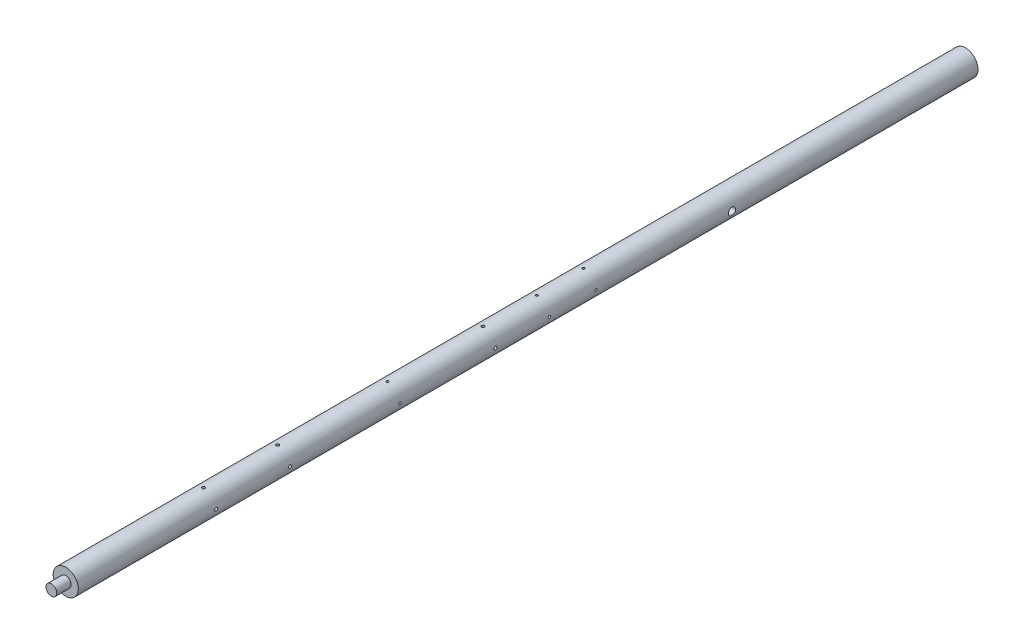
from build123d import *

# Parameters (mm, degrees)
SKETCH_1_R               = 17.5
EXTRUDE_1_DEPTH          = 1313
SKETCH_2_R               = 7.5
EXTRUDE_2_DEPTH          = 10
CHAMFER_1_SIZE           = 1
SKETCH_3_R               = 5
CUT_EXTRUDE_1_DEPTH      = 20
PATTERN_CIRCULAR_1_COUNT = 4
PATTERN_LINEAR_1_COUNT   = 2
PATTERN_LINEAR_1_PITCH   = 65
PATTERN_CIRCULAR_2_COUNT = 4
PATTERN_LINEAR_2_COUNT   = 2
PATTERN_LINEAR_2_PITCH   = 273
PATTERN_LINEAR_3_COUNT   = 2
PATTERN_LINEAR_3_PITCH   = 286
PATTERN_LINEAR_4_COUNT   = 2
PATTERN_LINEAR_4_PITCH   = 389
CUT_EXTRUDE_START        = -90
SKETCH_9_R               = 17.5
SKETCH_9_R_2             = 7.5
CUT_EXTRUDE_2_DEPTH      = 90
SKETCH_10_R              = 8.093395995
CUT_EXTRUDE_3_DEPTH      = 80
EXTRUDE_START            = 30
SKETCH_11_R              = 17.5
EXTRUDE_3_DEPTH          = 30


with BuildPart() as part:
    # 草图1 → 凸台-拉伸1 (new body)
    with BuildSketch(Plane.XY):
        Circle(SKETCH_1_R)
    extrude(amount=EXTRUDE_1_DEPTH)

    # 草图2 → 凸台-拉伸2 (add)
    with BuildSketch(Plane.XY.offset(1313)):
        Circle(SKETCH_2_R)
    extrude(amount=EXTRUDE_2_DEPTH)

    # 倒角1
    chamfer_1_edges = [part.edges().sort_by_distance(p)[0] for p in [
        (-7.5, 0, 1323),
    ]]
    chamfer(chamfer_1_edges, length=CHAMFER_1_SIZE)

    # 草图3 → 切除-拉伸1 (cut, symmetric)
    with BuildSketch(Plane(origin=(0, 0, 0), x_dir=(0, 0, -1), z_dir=(1, 0, 0))):
        with Locations(Location((-312.5, 0, 0), (0, 0, 180))):
            Circle(SKETCH_3_R)
    extrude(amount=CUT_EXTRUDE_1_DEPTH, both=True, mode=Mode.SUBTRACT)

    # 草图5 → M4x0.7 螺纹孔1 (revolve, cut)
    with BuildSketch(Plane(origin=(17.5, 0, 502), x_dir=(0, 0, -1), z_dir=(0, 1, 0))):
        Polygon((0, 0), (0, 11.091420021), (1.65, 10.1), (1.65, 0), align=None)
    m4x0_7_1 = revolve(axis=Axis((23.85, 0, 502), (-1, 0, 0)), mode=Mode.SUBTRACT)

    # 阵列(圆周)1: M4x0.7 螺纹孔1 ×4 about axis
    pattern_circular_1_axis = Axis((0, 0, 1313), (0, 0, -1))
    for i in range(1, PATTERN_CIRCULAR_1_COUNT):
        add(m4x0_7_1.rotate(pattern_circular_1_axis, i * 360 / PATTERN_CIRCULAR_1_COUNT), mode=Mode.SUBTRACT)

    # 阵列(线性)1: M4x0.7 螺纹孔1 ×2
    with Locations(*[(0, 0, i * PATTERN_LINEAR_1_PITCH) for i in range(1, PATTERN_LINEAR_1_COUNT)]):
        add(m4x0_7_1, mode=Mode.SUBTRACT)

    # 阵列(线性)1 copy 1 sketch → 阵列(线性)1 copy 1 (revolve, cut)
    with BuildSketch(Plane(origin=(0, -17.5, 567), x_dir=(0, 0, -1), z_dir=(1, 0, 0))):
        Polygon((0, 0), (0, 11.091420021), (1.65, 10.1), (1.65, 0), align=None)
    revolve(axis=Axis((0, -23.85, 567), (0, 1, 0)), mode=Mode.SUBTRACT)

    # 阵列(线性)1 copy 2 sketch → 阵列(线性)1 copy 2 (revolve, cut)
    with BuildSketch(Plane(origin=(-17.5, 0, 567), x_dir=(0, 0, -1), z_dir=(0, -1, 0))):
        Polygon((0, 0), (0, 11.091420021), (1.65, 10.1), (1.65, 0), align=None)
    revolve(axis=Axis((-23.85, 0, 567), (1, 0, 0)), mode=Mode.SUBTRACT)

    # 阵列(线性)1 copy 3 sketch → 阵列(线性)1 copy 3 (revolve, cut)
    with BuildSketch(Plane(origin=(0, 17.5, 567), x_dir=(0, 0, -1), z_dir=(-1, 0, 0))):
        Polygon((0, 0), (0, 11.091420021), (1.65, 10.1), (1.65, 0), align=None)
    revolve(axis=Axis((0, 23.85, 567), (0, -1, 0)), mode=Mode.SUBTRACT)

    # 草图8 → M5x0.8 螺纹孔1 (revolve, cut)
    with BuildSketch(Plane(origin=(17.5, 0, 642), x_dir=(0, 0, -1), z_dir=(0, 1, 0))):
        Polygon((0, 0), (0, 13.6618073), (2.1, 12.4), (2.1, 0), align=None)
    m5x0_8_1 = revolve(axis=Axis((23.85, 0, 642), (-1, 0, 0)), mode=Mode.SUBTRACT)

    # 阵列(圆周)2: M5x0.8 螺纹孔1 ×4 about axis
    pattern_circular_2_axis = Axis((0, 0, 1313), (0, 0, -1))
    for i in range(1, PATTERN_CIRCULAR_2_COUNT):
        add(m5x0_8_1.rotate(pattern_circular_2_axis, i * 360 / PATTERN_CIRCULAR_2_COUNT), mode=Mode.SUBTRACT)

    # 阵列(线性)2: M4x0.7 螺纹孔1 ×2
    with Locations(*[(0, 0, i * PATTERN_LINEAR_2_PITCH) for i in range(1, PATTERN_LINEAR_2_COUNT)]):
        add(m4x0_7_1, mode=Mode.SUBTRACT)

    # 阵列(线性)2 copy 1 sketch → 阵列(线性)2 copy 1 (revolve, cut)
    with BuildSketch(Plane(origin=(0, -17.5, 775), x_dir=(0, 0, -1), z_dir=(1, 0, 0))):
        Polygon((0, 0), (0, 11.091420021), (1.65, 10.1), (1.65, 0), align=None)
    revolve(axis=Axis((0, -23.85, 775), (0, 1, 0)), mode=Mode.SUBTRACT)

    # 阵列(线性)2 copy 2 sketch → 阵列(线性)2 copy 2 (revolve, cut)
    with BuildSketch(Plane(origin=(-17.5, 0, 775), x_dir=(0, 0, -1), z_dir=(0, -1, 0))):
        Polygon((0, 0), (0, 11.091420021), (1.65, 10.1), (1.65, 0), align=None)
    revolve(axis=Axis((-23.85, 0, 775), (1, 0, 0)), mode=Mode.SUBTRACT)

    # 阵列(线性)2 copy 3 sketch → 阵列(线性)2 copy 3 (revolve, cut)
    with BuildSketch(Plane(origin=(0, 17.5, 775), x_dir=(0, 0, -1), z_dir=(-1, 0, 0))):
        Polygon((0, 0), (0, 11.091420021), (1.65, 10.1), (1.65, 0), align=None)
    revolve(axis=Axis((0, 23.85, 775), (0, -1, 0)), mode=Mode.SUBTRACT)

    # 阵列(线性)3: M5x0.8 螺纹孔1 ×2
    with Locations(*[(0, 0, i * PATTERN_LINEAR_3_PITCH) for i in range(1, PATTERN_LINEAR_3_COUNT)]):
        add(m5x0_8_1, mode=Mode.SUBTRACT)

    # 阵列(线性)3 copy 1 sketch → 阵列(线性)3 copy 1 (revolve, cut)
    with BuildSketch(Plane(origin=(0, -17.5, 928), x_dir=(0, 0, -1), z_dir=(1, 0, 0))):
        Polygon((0, 0), (0, 13.6618073), (2.1, 12.4), (2.1, 0), align=None)
    revolve(axis=Axis((0, -23.85, 928), (0, 1, 0)), mode=Mode.SUBTRACT)

    # 阵列(线性)3 copy 2 sketch → 阵列(线性)3 copy 2 (revolve, cut)
    with BuildSketch(Plane(origin=(-17.5, 0, 928), x_dir=(0, 0, -1), z_dir=(0, -1, 0))):
        Polygon((0, 0), (0, 13.6618073), (2.1, 12.4), (2.1, 0), align=None)
    revolve(axis=Axis((-23.85, 0, 928), (1, 0, 0)), mode=Mode.SUBTRACT)

    # 阵列(线性)3 copy 3 sketch → 阵列(线性)3 copy 3 (revolve, cut)
    with BuildSketch(Plane(origin=(0, 17.5, 928), x_dir=(0, 0, -1), z_dir=(-1, 0, 0))):
        Polygon((0, 0), (0, 13.6618073), (2.1, 12.4), (2.1, 0), align=None)
    revolve(axis=Axis((0, 23.85, 928), (0, -1, 0)), mode=Mode.SUBTRACT)

    # 阵列(线性)4: M5x0.8 螺纹孔1 ×2
    with Locations(*[(0, 0, i * PATTERN_LINEAR_4_PITCH) for i in range(1, PATTERN_LINEAR_4_COUNT)]):
        add(m5x0_8_1, mode=Mode.SUBTRACT)

    # 阵列(线性)4 copy 1 sketch → 阵列(线性)4 copy 1 (revolve, cut)
    with BuildSketch(Plane(origin=(0, -17.5, 1031), x_dir=(0, 0, -1), z_dir=(1, 0, 0))):
        Polygon((0, 0), (0, 13.6618073), (2.1, 12.4), (2.1, 0), align=None)
    revolve(axis=Axis((0, -23.85, 1031), (0, 1, 0)), mode=Mode.SUBTRACT)

    # 阵列(线性)4 copy 2 sketch → 阵列(线性)4 copy 2 (revolve, cut)
    with BuildSketch(Plane(origin=(-17.5, 0, 1031), x_dir=(0, 0, -1), z_dir=(0, -1, 0))):
        Polygon((0, 0), (0, 13.6618073), (2.1, 12.4), (2.1, 0), align=None)
    revolve(axis=Axis((-23.85, 0, 1031), (1, 0, 0)), mode=Mode.SUBTRACT)

    # 阵列(线性)4 copy 3 sketch → 阵列(线性)4 copy 3 (revolve, cut)
    with BuildSketch(Plane(origin=(0, 17.5, 1031), x_dir=(0, 0, -1), z_dir=(-1, 0, 0))):
        Polygon((0, 0), (0, 13.6618073), (2.1, 12.4), (2.1, 0), align=None)
    revolve(axis=Axis((0, 23.85, 1031), (0, -1, 0)), mode=Mode.SUBTRACT)

    # 草图9 → 切除-拉伸2 (cut)
    with BuildSketch(Plane.XY.offset(1313).offset(CUT_EXTRUDE_START)):
        Circle(SKETCH_9_R)
        Circle(SKETCH_9_R_2, mode=Mode.SUBTRACT)
    extrude(amount=CUT_EXTRUDE_2_DEPTH, mode=Mode.SUBTRACT)

    # 草图10 → 切除-拉伸3 (cut)
    with BuildSketch(Plane.XY.offset(1323)):
        Circle(SKETCH_10_R)
    extrude(amount=-CUT_EXTRUDE_3_DEPTH, mode=Mode.SUBTRACT)

    # 草图11 → 凸台-拉伸3 (add)
    with BuildSketch(Plane(origin=(0, 0, 0), x_dir=(-1, 0, 0), z_dir=(0, 0, -1)).offset(EXTRUDE_START)):
        Circle(SKETCH_11_R)
    extrude(amount=-EXTRUDE_3_DEPTH)


solid = part.part
